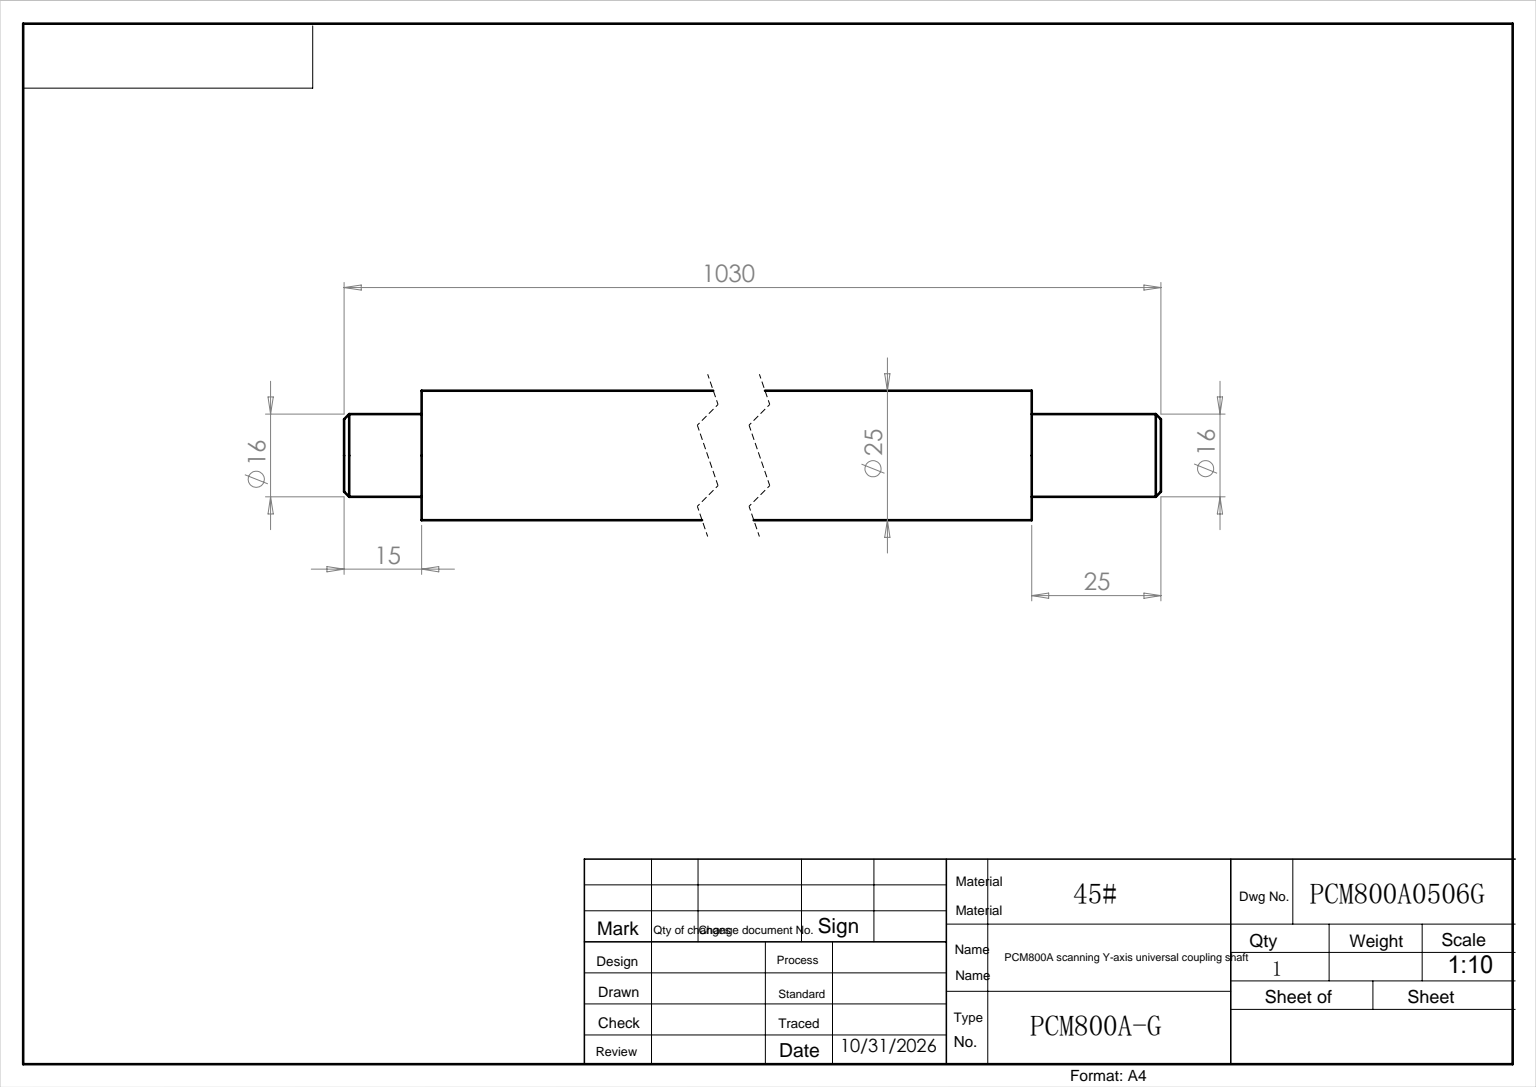
SolidWorks part; units mm, degrees
ref_plane "前视" through (0, 0, 0) normal (0, 0, 1) x (1, 0, 0)
ref_plane "上视" through (0, 0, 0) normal (0, 1, 0) x (1, 0, 0)
ref_plane "右视" through (0, 0, 0) normal (1, 0, 0) x (0, 0, -1)
sketch "草图1" plane through (0, 0, 0) normal (0, 0, 1) x (1, 0, 0)
  circle A0 centre (0, 0) radius 12.5
  dimension "D1" = 25
extrude "基体-拉伸" add sketch "草图1" along normal blind 990
sketch "草图2" plane through (0, 0, 990) normal (0, 0, 1) x (1, 0, 0)
  circle A0 centre (0, 0) radius 8
  dimension "D1" = 16
extrude "凸台-拉伸1" add sketch "草图2" along normal blind 15
sketch "草图3" plane through (0, 0, 0) normal (0, 0, -1) x (-1, 0, 0)
  circle A0 centre (0, 0) radius 8
  dimension "D1" = 16
extrude "凸台-拉伸2" add sketch "草图3" along normal blind 25
chamfer "倒角1" distance 1 angle 45 2 edges at (8, 0, 1005) (-8, 0, -25)
